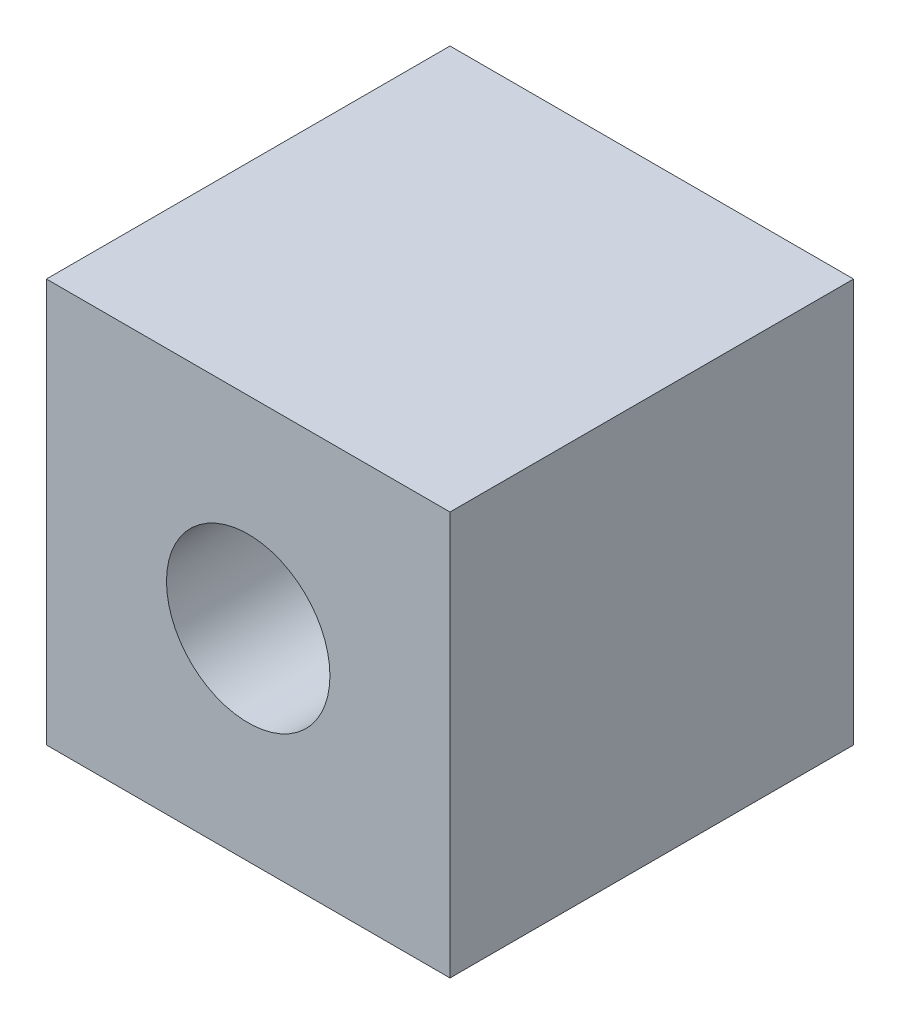
from build123d import *

# Parameters (mm, degrees)
SKETCH_1_W          = 40
SKETCH_1_H          = 40
EXTRUDE_1_DEPTH     = 20
SKETCH_2_R          = 8.1
CUT_EXTRUDE_1_DEPTH = 40


with BuildPart() as part:
    # 草图1 → 凸台-拉伸1 (new, symmetric)
    with BuildSketch(Plane.XY):
        Rectangle(SKETCH_1_W, SKETCH_1_H)
    extrude(amount=EXTRUDE_1_DEPTH, both=True)

    # 草图2 → 切除-拉伸1 (cut, symmetric)
    with BuildSketch(Plane.XY):
        Circle(SKETCH_2_R)
    extrude(amount=CUT_EXTRUDE_1_DEPTH, both=True, mode=Mode.SUBTRACT)


solid = part.part
